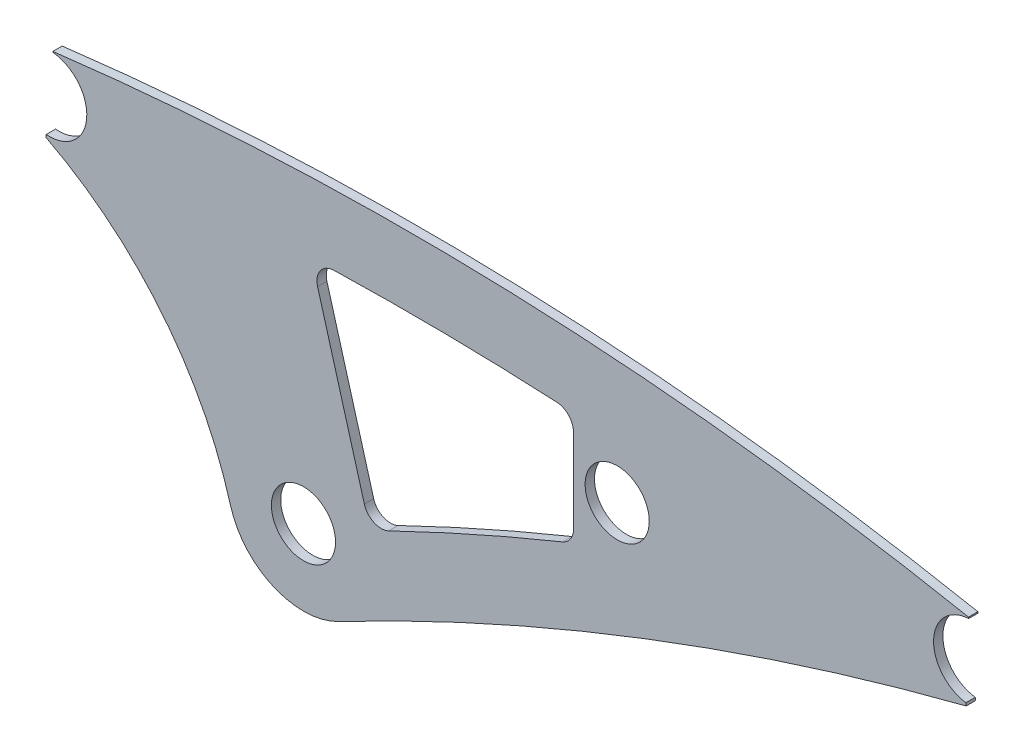
from build123d import *

# Parameters (mm, degrees)
SKETCH1_R           = 55
BOSS_EXTRUDE1_DEPTH = 16


with BuildPart() as part:
    # Sketch1 → Boss-Extrude1 (new body)
    with BuildSketch(Plane.XY):
        with BuildLine():
            Line((-441.486560332, 352.773302295), (-441.077967536, 357.443539322))
            ThreePointArc((-441.077967536, 357.443539322), (-371.743539322, 415.622032464), (-429.922032464, 484.956460678))
            Line((-429.922032464, 484.956460678), (-429.79492965, 486.409252487))
            ThreePointArc((-429.79492965, 486.409252487), (357.533978136, 521.031079354), (1140.522963582, 431.511647932))
            Line((1140.522963582, 431.511647932), (1140.708792797, 429.387610285))
            ThreePointArc((1140.708792797, 429.387610285), (1080.543840624, 367.868475852), (1135.99378326, 302.067797793))
            Line((1135.99378326, 302.067797793), (1136.4, 297.424719211))
            ThreePointArc((1136.4, 297.424719211), (586.381263284, 122.220397305), (60.221638572, -115.21004404))
            ThreePointArc((60.221638572, -115.21004404), (-51.454770489, -119.38344355), (-125.106294133, -35.332919047))
            ThreePointArc((-125.106294133, -35.332919047), (-243.082301892, 191.502339862), (-441.486560332, 352.773302295))
        make_face()
        Circle(SKETCH1_R, mode=Mode.SUBTRACT)
        with Locations((538, 300)):
            Circle(SKETCH1_R, mode=Mode.SUBTRACT)
        with BuildLine():
            Line((463, 367.628013441), (463, 222.86357491))
            ThreePointArc((463, 222.86357491), (457.896084334, 206.124847813), (444.32100101, 195.08165748))
            ThreePointArc((444.32100101, 195.08165748), (294.287770433, 131.138912095), (146.367210305, 62.450100371))
            ThreePointArc((146.367210305, 62.450100371), (121.015152193, 62.085681339), (104.438295549, 81.270766055))
            Line((104.438295549, 81.270766055), (24.221447422, 364.163456776))
            ThreePointArc((24.221447422, 364.163456776), (28.91122692, 390.115501396), (52.280902613, 402.336831507))
            ThreePointArc((52.280902613, 402.336831507), (243.460652484, 403.707205867), (434.547363171, 397.588081319))
            ThreePointArc((434.547363171, 397.588081319), (454.753400827, 388.286898998), (463, 367.628013441))
        make_face(mode=Mode.SUBTRACT)
    extrude(amount=BOSS_EXTRUDE1_DEPTH)


solid = part.part
